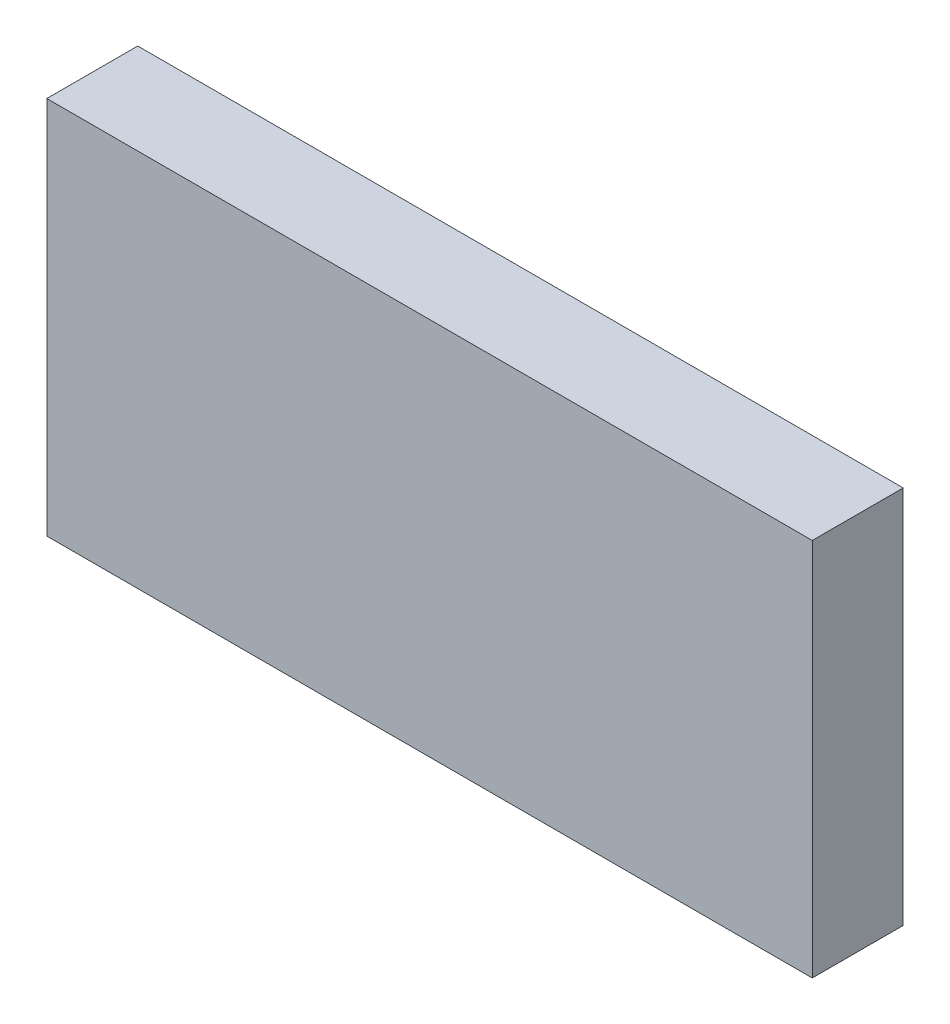
from build123d import *

# Parameters (mm, degrees)
SKETCH1_W           = 101
SKETCH1_H           = 50
BOSS_EXTRUDE1_DEPTH = 6


with BuildPart() as part:
    # Sketch1 → Boss-Extrude1 (new, symmetric)
    with BuildSketch(Plane.XY):
        Rectangle(SKETCH1_W, SKETCH1_H)
    extrude(amount=BOSS_EXTRUDE1_DEPTH, both=True)


solid = part.part
